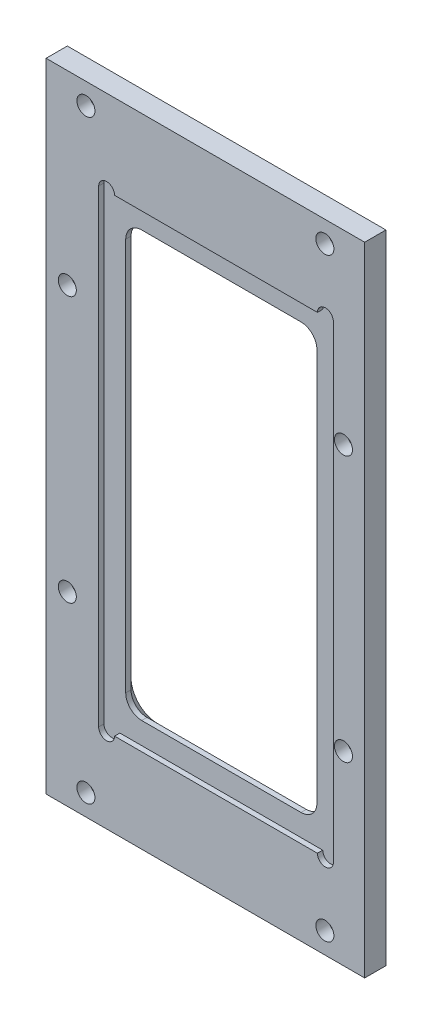
from build123d import *

# Parameters (mm, degrees)
SKETCH_1_W                   = 60
SKETCH_1_H                   = 120
EXTRUDE_1_DEPTH              = 2
SKETCH_2_W                   = 36
SKETCH_2_H                   = 80
CUT_EXTRUDE_1_DEPTH          = 68.201190466
SKETCH_3_W                   = 44.2
SKETCH_3_H                   = 88.2
CUT_EXTRUDE_2_DEPTH          = 1
HOLE_WIZARD_3_0_3_1_D        = 3
HOLE_WIZARD_3_0_3_1_DEPTH    = 1
FILLET_1_R                   = 3
CHAMFER_1_SIZE               = 2
HOLE_WIZARD_M3_1_D           = 3.4
HOLE_WIZARD_M3_1_CSINK_D     = 6.72
HOLE_WIZARD_M3_1_CSINK_ANGLE = 90


with BuildPart() as part:
    # 草图1 → 凸台-拉伸1 (new, symmetric)
    with BuildSketch(Plane.XY):
        Rectangle(SKETCH_1_W, SKETCH_1_H)
    extrude(amount=EXTRUDE_1_DEPTH, both=True)

    # 草图2 → 切除-拉伸1 (cut, through all)
    with BuildSketch(Plane.XY.offset(2)):
        with Locations((2, 0)):
            Rectangle(SKETCH_2_W, SKETCH_2_H)
    extrude(amount=-CUT_EXTRUDE_1_DEPTH, mode=Mode.SUBTRACT)

    # 草图3 → 切除-拉伸2 (cut)
    with BuildSketch(Plane.XY.offset(2)):
        with Locations((2, 0)):
            Rectangle(SKETCH_3_W, SKETCH_3_H)
    extrude(amount=-CUT_EXTRUDE_2_DEPTH, mode=Mode.SUBTRACT)

    # Ø3.0 (3) 直径孔1
    with Locations(Plane.XY.offset(2)):
        with Locations((-18.6, 44.1), (22.6, 44.1), (22.6, -44.1), (-18.6, -44.1)):
            Hole(HOLE_WIZARD_3_0_3_1_D / 2, depth=HOLE_WIZARD_3_0_3_1_DEPTH)

    # 圆角1
    fillet_1_edges = [part.edges().sort_by_distance(p)[0] for p in [
        (-16, -40, -0.5),
        (-16, 40, -0.5),
        (20, 40, -0.5),
        (20, -40, -0.5),
    ]]
    fillet(fillet_1_edges, radius=FILLET_1_R)

    # 倒角1
    chamfer_1_edges = [part.edges().sort_by_distance(p)[0] for p in [
        (20, 0, -2),
        (2, -40, -2),
        (-16, 0, -2),
        (19.121320344, 39.121320344, -2),
        (19.121320344, -39.121320344, -2),
        (-15.121320344, -39.121320344, -2),
        (-15.121320344, 39.121320344, -2),
        (2, 40, -2),
    ]]
    chamfer(chamfer_1_edges, length=CHAMFER_1_SIZE)

    # M3 六角凹锥坑螺钉的锥形沉头孔1 (through all)
    with Locations(Plane(origin=(0, 0, -2), x_dir=(-1, 0, 0), z_dir=(0, 0, -1))):
        with Locations((-22.5, 56), (22.5, 56), (26, 25), (26, -25), (22.5, -56), (-22.5, -56), (-26, -25), (-26, 25)):
            CounterSinkHole(HOLE_WIZARD_M3_1_D / 2, HOLE_WIZARD_M3_1_CSINK_D / 2, counter_sink_angle=HOLE_WIZARD_M3_1_CSINK_ANGLE)


solid = part.part
